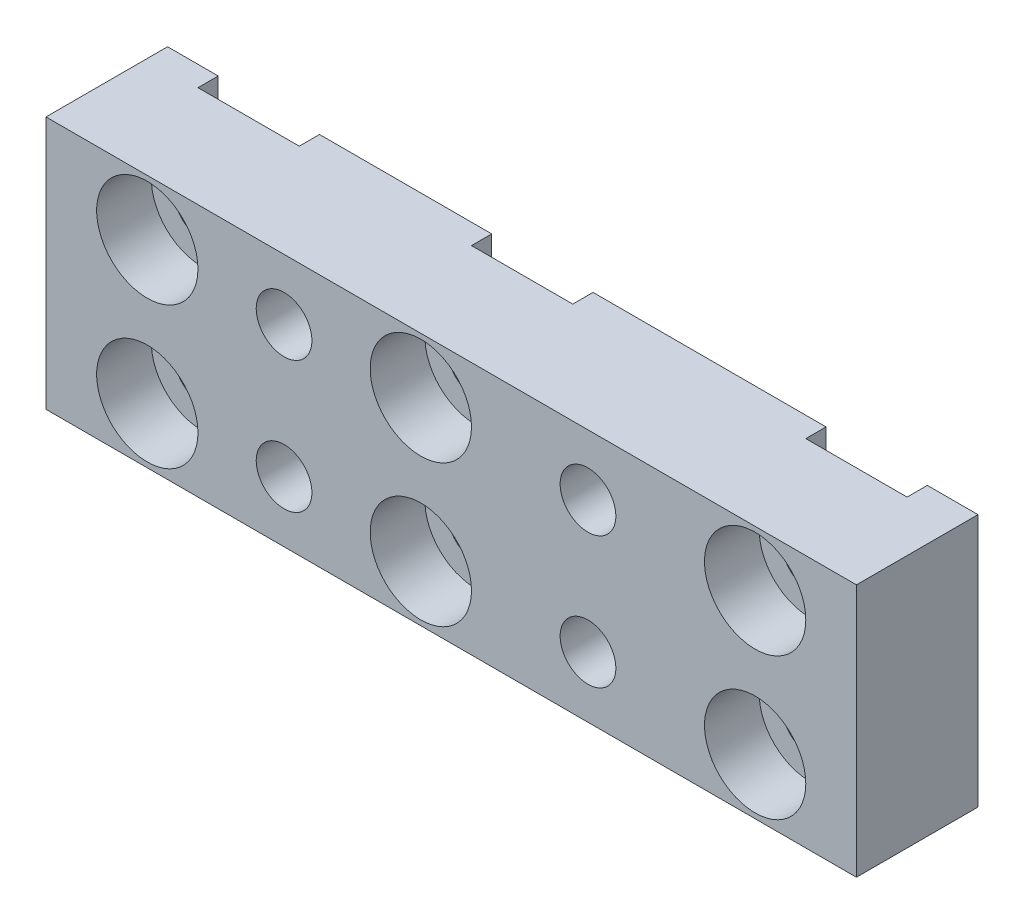
from build123d import *

# Parameters (mm, degrees)
SKETCH1_W                                           = 80
SKETCH1_H                                           = 25
BOSS_EXTRUDE1_DEPTH                                 = 12
SKETCH2_W                                           = 10
SKETCH2_H                                           = 2
CUT_EXTRUDE1_DEPTH                                  = 49.672374095
CBORE_FOR_M5_HEX_SOCKET_HEAD_CAP_SCREW1_D           = 5.5
CBORE_FOR_M5_HEX_SOCKET_HEAD_CAP_SCREW1_CBORE_D     = 10
CBORE_FOR_M5_HEX_SOCKET_HEAD_CAP_SCREW1_CBORE_DEPTH = 5.4
CBORE_FOR_M5_HEX_SOCKET_HEAD_CAP_SCREW2_D           = 5.5
CBORE_FOR_M5_HEX_SOCKET_HEAD_CAP_SCREW2_CBORE_D     = 10
CBORE_FOR_M5_HEX_SOCKET_HEAD_CAP_SCREW2_CBORE_DEPTH = 5.4


with BuildPart() as part:
    # Sketch1 → Boss-Extrude1 (new body)
    with BuildSketch(Plane.XY):
        Rectangle(SKETCH1_W, SKETCH1_H)
    extrude(amount=BOSS_EXTRUDE1_DEPTH)

    # Sketch2 → Cut-Extrude1 (cut, through all)
    with BuildSketch(Plane(origin=(0, 12.5, 0), x_dir=(1, 0, 0), z_dir=(0, 1, 0))):
        with Locations((-30, -1)):
            Rectangle(SKETCH2_W, SKETCH2_H)
        with Locations((-3, -1)):
            Rectangle(SKETCH2_W, SKETCH2_H)
        with Locations((30, -1)):
            Rectangle(SKETCH2_W, SKETCH2_H)
    extrude(amount=-CUT_EXTRUDE1_DEPTH, mode=Mode.SUBTRACT)

    # CBORE for M5 Hex Socket Head Cap Screw1 (through all)
    with Locations(Plane.XY.offset(12)):
        with Locations((-30, 7), (-30, -7), (-3, 7), (-3, -7), (30, 7), (30, -7)):
            CounterBoreHole(CBORE_FOR_M5_HEX_SOCKET_HEAD_CAP_SCREW1_D / 2, CBORE_FOR_M5_HEX_SOCKET_HEAD_CAP_SCREW1_CBORE_D / 2, CBORE_FOR_M5_HEX_SOCKET_HEAD_CAP_SCREW1_CBORE_DEPTH)

    # CBORE for M5 Hex Socket Head Cap Screw2 (through all)
    with Locations(Plane(origin=(0, 0, 0), x_dir=(-1, 0, 0), z_dir=(0, 0, -1))):
        with Locations((-13.5, 6.5), (-13.5, -6.5), (16.5, 6.5), (16.5, -6.5)):
            CounterBoreHole(CBORE_FOR_M5_HEX_SOCKET_HEAD_CAP_SCREW2_D / 2, CBORE_FOR_M5_HEX_SOCKET_HEAD_CAP_SCREW2_CBORE_D / 2, CBORE_FOR_M5_HEX_SOCKET_HEAD_CAP_SCREW2_CBORE_DEPTH)


solid = part.part
